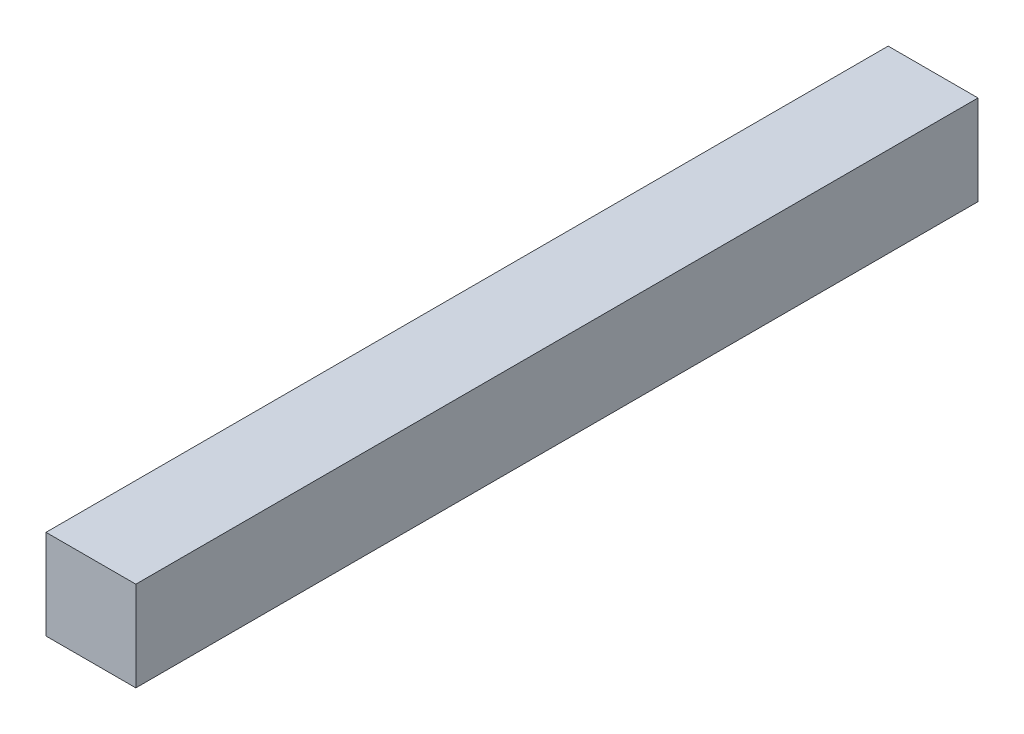
SolidWorks part; units mm, degrees
material "1023 碳钢板 (SS)"
ref_plane "前视基准面" through (0, 0, 0) normal (0, 0, 1) x (1, 0, 0)
ref_plane "上视基准面" through (0, 0, 0) normal (0, 1, 0) x (1, 0, 0)
ref_plane "右视基准面" through (0, 0, 0) normal (1, 0, 0) x (0, 0, -1)
sketch "草图1" plane through (0, 0, 0) normal (0, 0, 1) x (1, 0, 0)
  line L1 (8, 8) -> (-8, 8)
  line L2 (8, 8) -> (8, -8)
  line L3 (8, -8) -> (-8, -8)
  line L4 (-8, 8) -> (-8, -8)
  line L5 (8, 8) -> (-8, -8) construction
  line L6 (8, -8) -> (-8, 8) construction
  point P0 (0, 0)
  dimension "D1" = 16
  dimension "D2" = 16
extrude "凸台-拉伸1" add sketch "草图1" along normal blind 150
